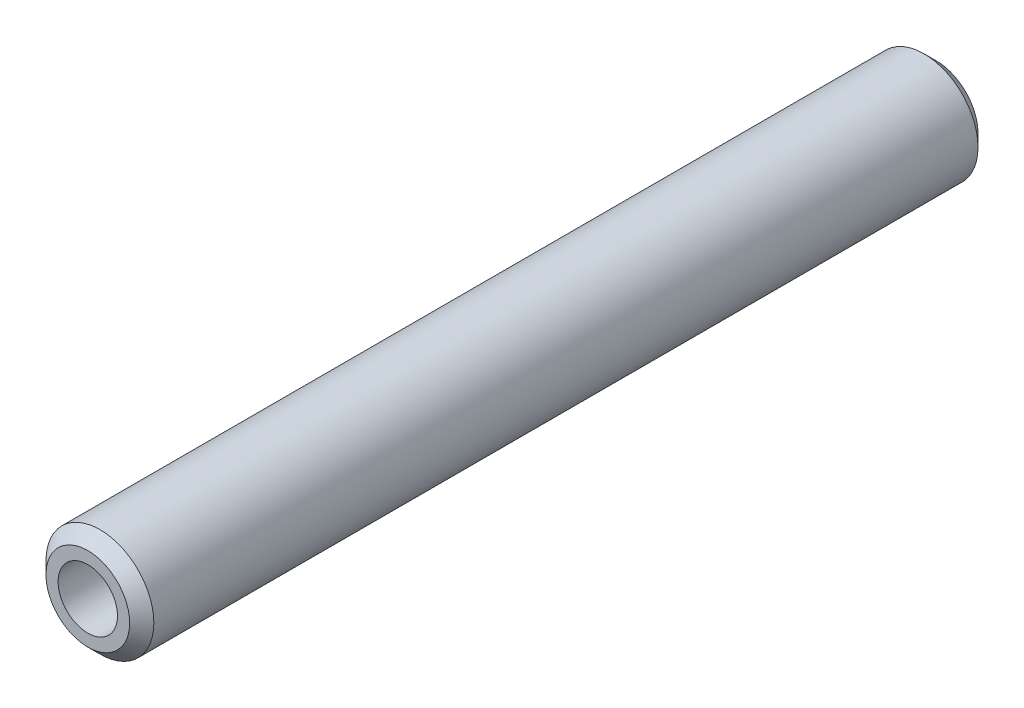
SolidWorks part; units mm, degrees
material "普通碳钢"
ref_plane "Front Plane" through (0, 0, 0) normal (0, 0, 1) x (1, 0, 0)
ref_plane "Top Plane" through (0, 0, 0) normal (0, 1, 0) x (1, 0, 0)
ref_plane "Right Plane" through (0, 0, 0) normal (1, 0, 0) x (0, 0, -1)
sketch "Sketch1" plane through (0, 0, 0) normal (0, 0, 1) x (1, 0, 0)
  circle A0 centre (0, 0) radius 44.5
  dimension "D1" = 89
extrude "Extrude-Thin1" add sketch "Sketch1" along normal mid plane 700 thin thin type one direction reverse wall 20
chamfer "Chamfer1" distance 10 angle 45 2 edges at (44.5, 0, 350) (44.5, 0, -350)
